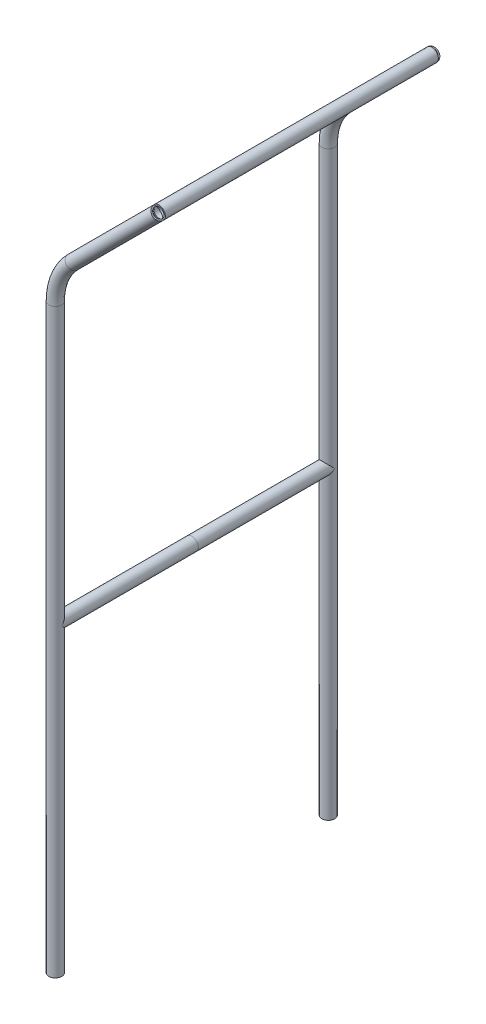
from build123d import *

# Parameters (mm, degrees)
SKETCH1_ON_SEGMENT_1_R    = 10.65
SKETCH1_ON_SEGMENT_1_R_2  = 8.35
PIPE_21_3_X_2_3_1_DEPTH   = 958.578643763
SKETCH1_ON_SEGMENT_2_R    = 10.65
SKETCH1_ON_SEGMENT_2_R_2  = 8.35
PIPE_21_3_X_2_3_1_2_ANGLE = 45
SKETCH1_R                 = 10.65
SKETCH1_R_2               = 8.35
PIPE_21_3_X_2_3_1_3_DEPTH = 200
SKETCH11_R                = 10.65
SKETCH11_R_2              = 8.35
PIPE_21_3_X_2_3_2_DEPTH   = 225
SKETCH12_R                = 10.65
SKETCH12_R_2              = 8.35
PIPE_21_3_X_2_3_3_DEPTH   = 450


with BuildPart() as part:
    # Sketch1 on segment 1 (carried to segment 1) → Pipe 21.3 X 2.3(1) (new body)
    with BuildSketch(Plane(origin=(0, -500, 0), x_dir=(-1, 0, 0), z_dir=(0, 1, 0))):
        Circle(SKETCH1_ON_SEGMENT_1_R)
        Circle(SKETCH1_ON_SEGMENT_1_R_2, mode=Mode.SUBTRACT)
    extrude(amount=PIPE_21_3_X_2_3_1_DEPTH)


with BuildPart() as body_2:
    # Sketch1 on segment 2 (carried to the start of arc 2) → Pipe 21.3 X 2.3_1 2 (revolve)
    with BuildSketch(Plane(origin=(29.289321881, 529.289321881, 0), x_dir=(0.707106781, -0.707106781, 0), z_dir=(-0.707106781, -0.707106781, 0))):
        Circle(SKETCH1_ON_SEGMENT_2_R)
        Circle(SKETCH1_ON_SEGMENT_2_R_2, mode=Mode.SUBTRACT)
    revolve(axis=Axis((100, 458.578643763, 0), (0, 0, 1)), revolution_arc=PIPE_21_3_X_2_3_1_2_ANGLE)


with BuildPart() as body_3:
    # Sketch1 → Pipe 21.3 X 2.3_1 3 (new body)
    with BuildSketch(Plane(origin=(29.289321881, 529.289321881, 0), x_dir=(-0.7071067811865461, 0.7071067811865489, 0), z_dir=(0.7071067811865489, 0.7071067811865461, 0))):
        Circle(SKETCH1_R)
        Circle(SKETCH1_R_2, mode=Mode.SUBTRACT)
    extrude(amount=PIPE_21_3_X_2_3_1_3_DEPTH)


with BuildPart() as body_4:
    # Sketch11 → Pipe 21.3 X 2.3(2) (new body)
    with BuildSketch(Plane(origin=(0, 0, 0), x_dir=(0, -1, 0), z_dir=(0, 0, 1))):
        Circle(SKETCH11_R)
        Circle(SKETCH11_R_2, mode=Mode.SUBTRACT)
    extrude(amount=PIPE_21_3_X_2_3_2_DEPTH)


with BuildPart() as body_5:
    # Mirror1: mirrored copy
    add(body_3.part.mirror(Plane.XY.offset(225)))


with BuildPart() as body_6:
    # Mirror1 2: mirrored copy
    add(body_2.part.mirror(Plane.XY.offset(225)))


with BuildPart() as body_7:
    # Mirror1 3: mirrored copy
    add(part.part.mirror(Plane.XY.offset(225)))


with BuildPart() as body_8:
    # Mirror1 4: mirrored copy
    add(body_4.part.mirror(Plane.XY.offset(225)))


with BuildPart() as body_9:
    # Sketch12 → Pipe 21.3 X 2.3(3) (new body)
    with BuildSketch(Plane(origin=(170.710678119, 670.710678119, 450), x_dir=(-0.7071067811865461, 0.7071067811865489, 0), z_dir=(0, 0, -1))):
        Circle(SKETCH12_R)
        Circle(SKETCH12_R_2, mode=Mode.SUBTRACT)
    extrude(amount=PIPE_21_3_X_2_3_3_DEPTH)


solid = Compound([part.part, body_2.part, body_3.part, body_4.part, body_5.part, body_6.part, body_7.part, body_8.part, body_9.part])
